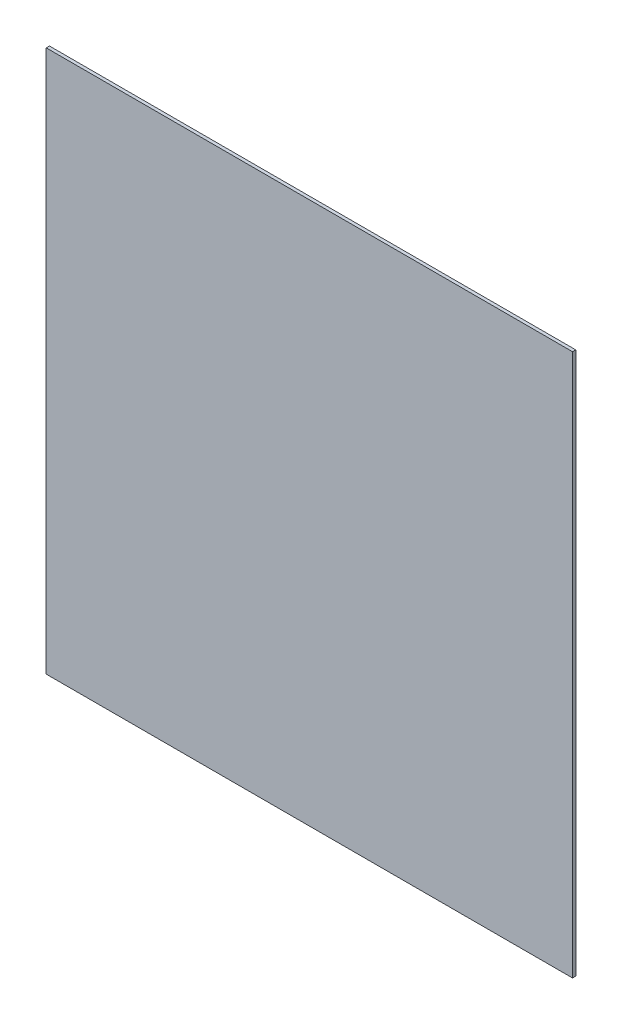
SolidWorks part; units mm, degrees
material "PMMA(有机玻璃)"
ref_plane "前视" through (0, 0, 0) normal (0, 0, 1) x (1, 0, 0)
ref_plane "上视" through (0, 0, 0) normal (0, 1, 0) x (1, 0, 0)
ref_plane "右视" through (0, 0, 0) normal (1, 0, 0) x (0, 0, -1)
sketch "草图1" plane through (0, 0, 0) normal (0, 0, 1) x (1, 0, 0)
  line L1 (-408.5, 421) -> (408.5, 421)
  line L2 (-408.5, 421) -> (-408.5, -421)
  line L3 (-408.5, -421) -> (408.5, -421)
  line L4 (408.5, 421) -> (408.5, -421)
  line L5 (-408.5, 421) -> (408.5, -421) construction
  line L6 (-408.5, -421) -> (408.5, 421) construction
  point P0 (0, 0)
  dimension "D1" = 842
  dimension "D2" = 817
extrude "凸台-拉伸1" add sketch "草图1" along normal blind 5
hole_wizard "M5 间隙孔1" positions "草图3" profile "草图2" hole size "M5" standard "GB"
sketch "草图3" plane through (0, 0, 5) normal (0, 0, 1) x (1, 0, 0)
  line L0 (-427.5, 273) -> (-427.5, -273) construction
  line L1 (-427.5, -273) -> (427.5, -273) construction
  line L2 (0, 273) -> (0, -273) construction
  line L3 (427.5, 273) -> (-427.5, 273) construction
  line L5 (-427.5, 0) -> (427.5, 0) construction
  line L6 (427.5, -273) -> (427.5, 273) construction
  point P0 (-375, -261)
  point P46 (415.5, 250)
  point P48 (-415.5, 250)
  point P58 (-125, -261)
  point P59 (125, -261)
  point P61 (-125, 261)
  point P62 (125, 261)
  point P64 (-375, 261)
  point P88 (375, -261)
  point P89 (375, 261)
  point P108 (415.5, 0)
  point P109 (-415.5, 0)
  point P110 (415.5, -250)
  point P111 (-415.5, -250)
  dimension "D1" = 12
  dimension "D2" = 12
  dimension "D5" = 3
  dimension "D3" = 12
  dimension "D6" = 4
  dimension "D4" = 2
sketch "草图2" plane through (-375, -261, 5) normal (1, 0, 0) x (0, -1, 0)
  line L0 (0, 0) -> (0, 5)
  line L1 (0, 5) -> (2.75, 5)
  line L2 (2.75, 5) -> (2.75, 0)
  line L5 (2.75, 0) -> (0, 0)
  line L11 (0, -6.35) -> (0, 107.95) construction
  dimension "通孔孔直径" = 5.5
  dimension "通孔孔深度" = 5
